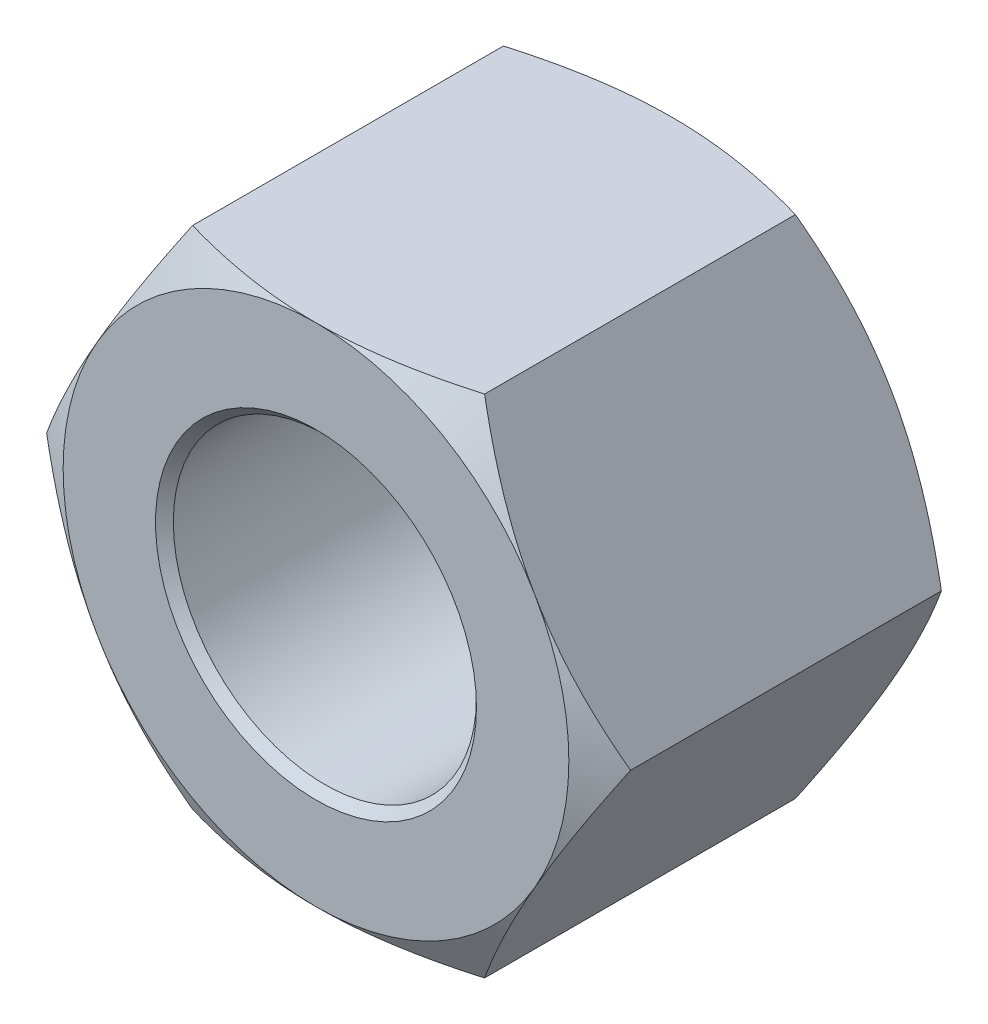
SolidWorks part; units mm, degrees
material "Q235"
ref_plane "Plane1" through (0, 0, 0) normal (0, 0, 1) x (1, 0, 0)
ref_plane "Plane2" through (0, 0, 0) normal (0, 1, 0) x (1, 0, 0)
ref_plane "Plane3" through (0, 0, 0) normal (1, 0, 0) x (0, 0, -1)
sketch "Dimension Sketch" plane through (0, 0, 0) normal (0, 0, 1) x (1, 0, 0)
  line L0 (0, 0) -> (21, 0) construction
  point P1 (19.2, 0)
  point P3 (14, 0)
  point P4 (2, 0)
  point P5 (22.8, 0)
  point P6 (13.9, 0)
  point P8 (21, 0)
  dimension "D" = 14
  dimension "e(最小)" = 22.8
  dimension "m(最大)" = 13.9
  dimension "s(公称)" = 21
  dimension "dw(最小)" = 19.2
  dimension "P" = 2
sketch "Sketch1" plane through (0, 0, 0) normal (0, 0, 1) x (1, 0, 0)
  line L0 (-26.8088, 0) -> (37.1748, 0) construction
  line L1 (0, 25.0215) -> (0, -25.0215) construction
  line L3 (5.7, 9.8727) -> (-5.7, 9.8727)
  line L4 (-5.7, 9.8727) -> (-11.4, 0)
  line L5 (-11.4, 0) -> (-5.7, -9.8727)
  line L6 (-5.7, -9.8727) -> (5.7, -9.8727)
  line L7 (5.7, -9.8727) -> (11.4, 0)
  line L8 (11.4, 0) -> (5.7, 9.8727)
  circle A0 centre (0, 0) radius 9.8727 construction
  circle A1 centre (0, 0) radius 5.9175
  dimension "D" = 11.835
  dimension "e" = 22.8
extrude "Boss-Extrude" add sketch "Sketch1" along normal blind 13.9
cosmetic thread "Cosmetic Thread1" parameters "D2"=14
sketch "Sketch2" plane through (0, 0, 0) normal (0, 0, -1) x (-1, 0, 0)
  line L0 (-5.7, 9.8727) -> (5.7, 9.8727) construction
  circle A0 centre (0, 0) radius 9.8727
  circle A1 centre (0, 0) radius 5.9175 construction
extrude "Cut-Extrude1" cut sketch "Sketch2" against normal through all draft 60 flip side to cut
sketch "Sketch3" plane through (0, 0, 13.9) normal (0, 0, 1) x (1, 0, 0)
  line L0 (11.4, 0) -> (5.7, 9.8727) construction
  circle A0 centre (0, 0) radius 9.8727
extrude "Cut-Extrude2" cut sketch "Sketch3" against normal through all draft 60 flip side to cut
chamfer "Chamfer1" distance 0.3475 angle 45 2 edges at (5.9175, 0, 0) (5.9175, 0, 13.9)
